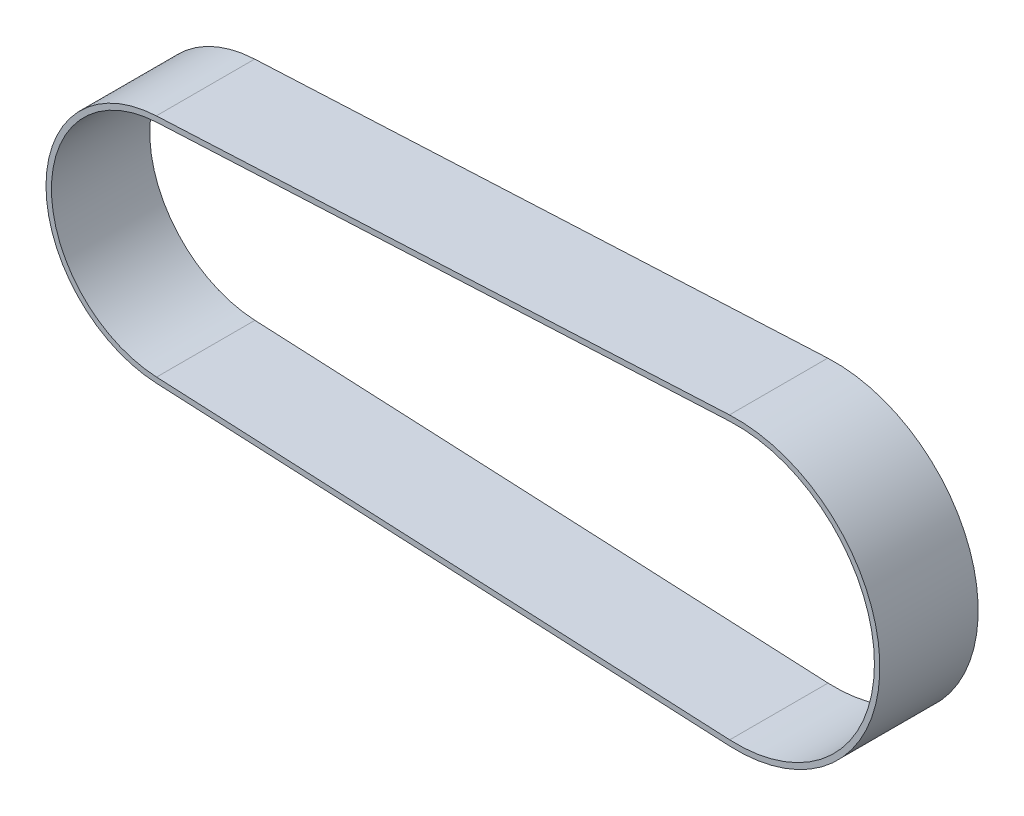
from build123d import *

# Parameters (mm, degrees)
BOSS_EXTRUDE1_DEPTH = 35.6


with BuildPart() as part:
    # Sketch1 → Boss-Extrude1 (new body)
    with BuildSketch(Plane.XY):
        with BuildLine():
            Line((-2.017486069, 41.915184916), (205.5017447, 51.903621277))
            ThreePointArc((205.5017447, 51.903621277), (259.963710234, 0), (205.5017447, -51.903621277))
            Line((205.5017447, -51.903621277), (-2.017486069, -41.915184916))
            ThreePointArc((-2.017486069, -41.915184916), (-41.963710234, 0), (-2.017486069, 41.915184916))
        make_face()
        with BuildLine():
            Line((-1.923076923, 39.953745446), (205.596153846, 49.942181807))
            ThreePointArc((205.596153846, 49.942181807), (258, 0), (205.596153846, -49.942181807))
            Line((205.596153846, -49.942181807), (-1.923076923, -39.953745446))
            ThreePointArc((-1.923076923, -39.953745446), (-40, 0), (-1.923076923, 39.953745446))
        make_face(mode=Mode.SUBTRACT)
    extrude(amount=BOSS_EXTRUDE1_DEPTH)


solid = part.part
